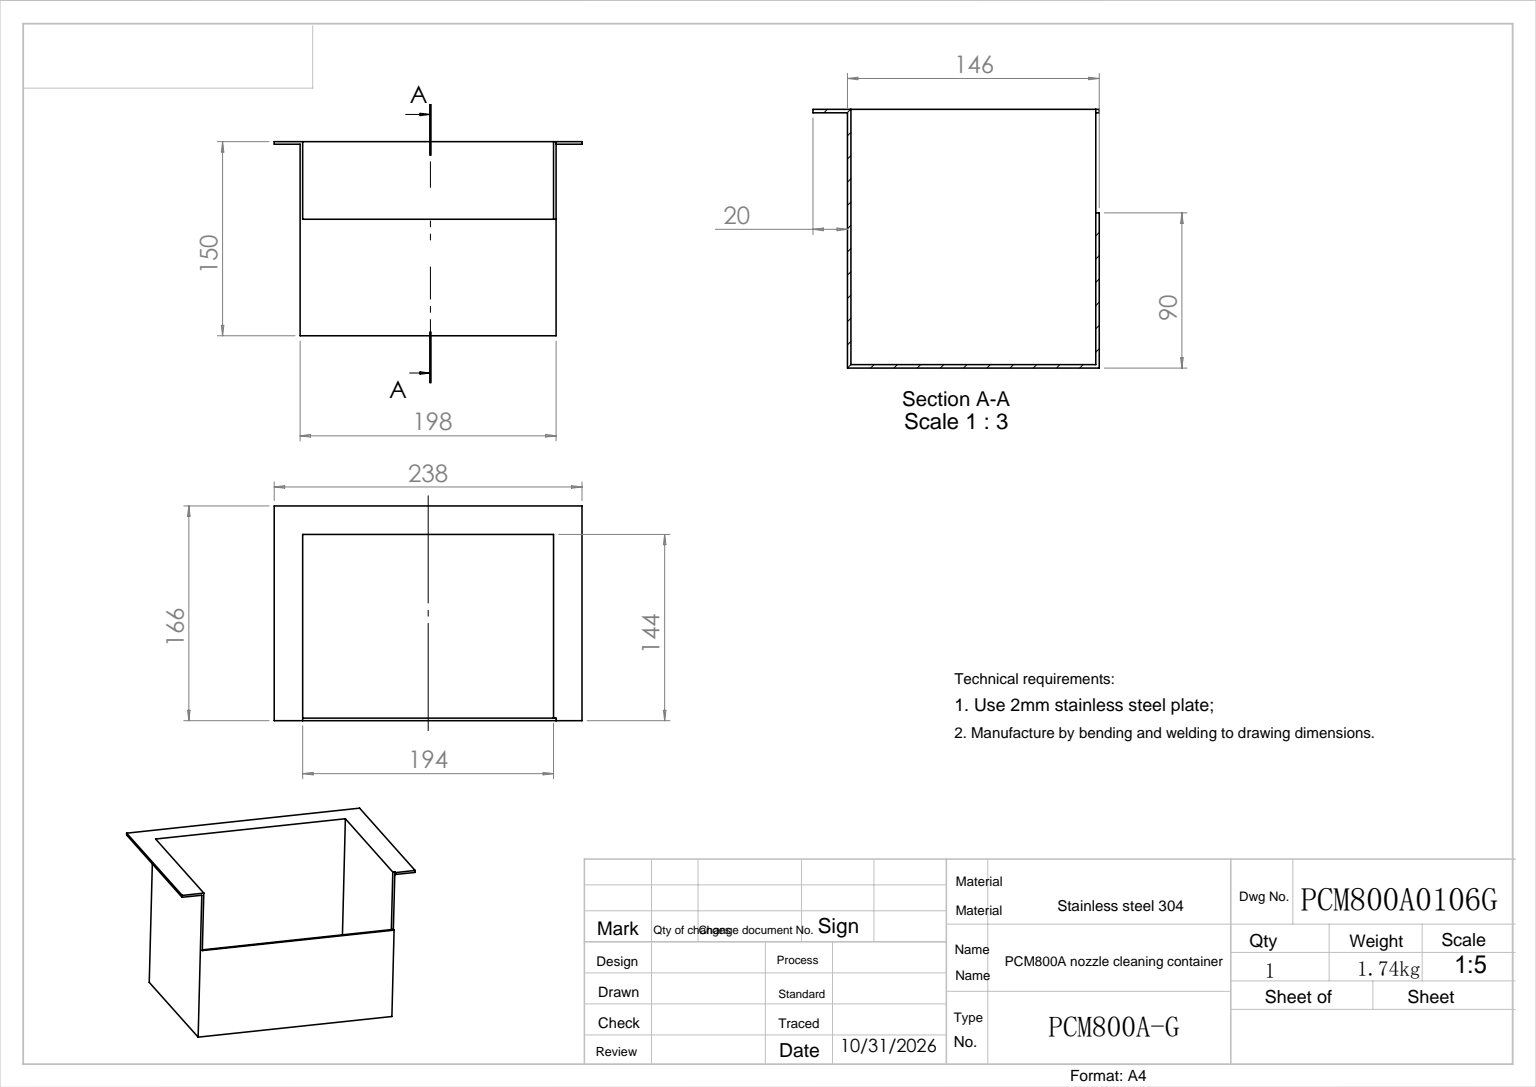
from build123d import *

# Parameters (mm, degrees)
SKETCH_1_W          = 198
SKETCH_1_H          = 146
EXTRUDE_1_DEPTH     = 150
SHELL_1_T           = -2
EXTRUDE_2_DEPTH     = 2
SKETCH_3_W          = 196
SKETCH_3_H          = 60
CUT_EXTRUDE_1_DEPTH = 2


with BuildPart() as part:
    # 草图1 → 凸台-拉伸1 (new body)
    with BuildSketch(Plane.XY):
        with Locations((99, -73)):
            Rectangle(SKETCH_1_W, SKETCH_1_H)
    extrude(amount=EXTRUDE_1_DEPTH)

    # 抽壳1
    shell_1_openings = [part.faces().sort_by_distance(p)[0] for p in [
        (99, -73, 150),
    ]]
    offset(amount=SHELL_1_T, openings=shell_1_openings, kind=Kind.INTERSECTION)

    # 草图2 → 凸台-拉伸2 (add)
    with BuildSketch(Plane.XY.offset(150)):
        Polygon((0, -146), (-20, -146), (-20, 20), (218, 20), (218, -146), (198, -146), (198, 0), (0, 0), align=None)
    extrude(amount=-EXTRUDE_2_DEPTH)

    # 草图3 → 切除-拉伸1 (cut)
    with BuildSketch(Plane.XZ.offset(146)):
        with Locations((100, 120)):
            Rectangle(SKETCH_3_W, SKETCH_3_H)
    extrude(amount=-CUT_EXTRUDE_1_DEPTH, mode=Mode.SUBTRACT)


solid = part.part
